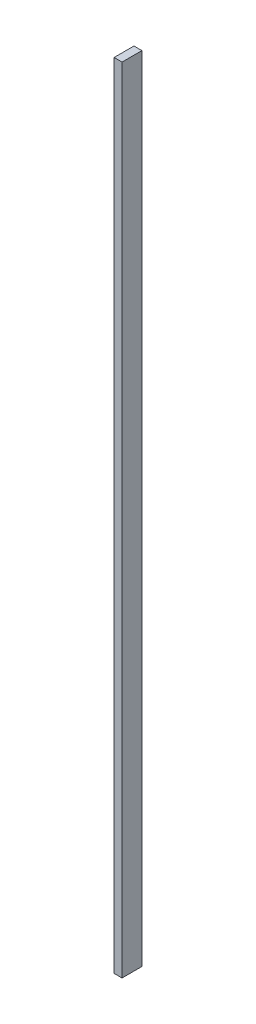
from build123d import *

# Parameters (mm, degrees)
SKETCH1_W           = 50
SKETCH1_H           = 1996
BOSS_EXTRUDE1_DEPTH = 20


with BuildPart() as part:
    # Sketch1 → Boss-Extrude1 (new body)
    with BuildSketch(Plane(origin=(0, 0, 0), x_dir=(0, 0, -1), z_dir=(1, 0, 0))):
        with Locations((25, 998)):
            Rectangle(SKETCH1_W, SKETCH1_H)
    extrude(amount=BOSS_EXTRUDE1_DEPTH)


solid = part.part
